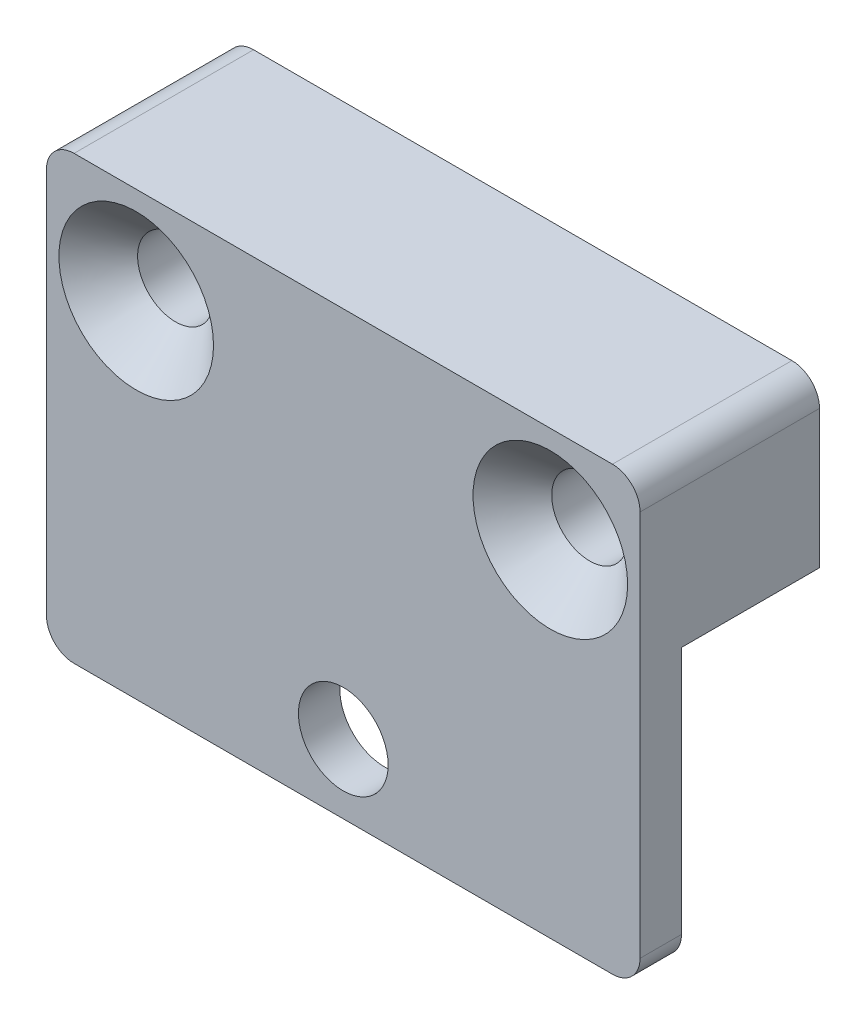
SolidWorks part; units mm, degrees
ref_plane "前视" through (0, 0, 0) normal (0, 0, 1) x (1, 0, 0)
ref_plane "上视" through (0, 0, 0) normal (0, 1, 0) x (1, 0, 0)
ref_plane "右视" through (0, 0, 0) normal (1, 0, 0) x (0, 0, -1)
sketch "草图1" plane through (0, 0, 0) normal (0, 0, 1) x (1, 0, 0)
  line L1 (0, 0) -> (43, 0)
  line L2 (0, 0) -> (0, -32)
  line L3 (0, -32) -> (43, -32)
  line L4 (43, 0) -> (43, -32)
  dimension "D1" = 43
  dimension "D2" = 32
extrude "凸台-拉伸1" add sketch "草图1" along normal blind 3
hole_wizard "M5 六角凹锥坑螺钉的锥形沉头孔1" positions "草图3" profile "草图2" countersink size "M5" standard "ISO" end condition through all
sketch "草图3" plane through (0, 0, 3) normal (0, 0, 1) x (1, 0, 0)
  line L0 (6.5, -7) -> (36.5, -7) construction
  line L2 (21.5, -7) -> (21.5, 0) construction
  line L3 (43, 0) -> (0, 0) construction
  point P0 (6.5, -7)
  point P2 (36.5, -7)
  dimension "D1" = 30
  dimension "D2" = 7
sketch "草图2" plane through (6.5, -7, 3) normal (1, 0, 0) x (0, -1, 0)
  line L0 (0, 0) -> (0, 3)
  line L1 (0, 3) -> (2.75, 3)
  line L2 (2.75, 3) -> (2.75, 2.85)
  line L3 (2.75, 2.85) -> (5.6, 0)
  line L5 (5.6, 0) -> (0, 0)
  line L6 (-2.75, 2.85) -> (-5.6, 0) construction
  line L11 (0, -6.35) -> (0, 107.95) construction
  dimension "通孔孔直径" = 5.5
  dimension "通孔孔深度" = 3
  dimension "近端锥形沉头孔直径" = 11.2
  dimension "近端锥形沉头孔角度" = 90
sketch "草图4" plane through (0, 0, 3) normal (0, 0, 1) x (1, 0, 0)
  line L0 (21.5, -32) -> (21.5, -27) construction
  line L1 (0, -32) -> (43, -32) construction
  circle A0 centre (21.5, -27) radius 3.25
  circle A1 centre (36.5, -7) radius 2.75 construction
  dimension "D1" = 6.5
  dimension "D2" = 20
extrude "切除-拉伸1" cut sketch "草图4" against normal blind 3
fillet "圆角1" radius 2 4 edges at (43, -32, 1.5) (0, -32, 1.5) (43, 0, 1.5) (0, 0, 1.5)
sketch "草图5" plane through (0, 0, 0) normal (0, 0, -1) x (-1, 0, 0)
  line L0 (-43, -12) -> (0, -12)
  line L4 (-2, 0) -> (-41, 0)
  line L5 (-43, -2) -> (-43, -30)
  line L6 (-41, -32) -> (-2, -32)
  line L7 (0, -30) -> (0, -2)
  line L8 (-2, 0) -> (-41, 0)
  line L9 (-43, -2) -> (-43, -30)
  line L10 (-41, -32) -> (-2, -32)
  line L11 (0, -30) -> (0, -2)
  arc A4 (-41, 0) -> (-43, -2) centre (-41, -2) ccw
  arc A5 (-43, -30) -> (-41, -32) centre (-41, -30) ccw
  arc A6 (-2, -32) -> (0, -30) centre (-2, -30) ccw
  arc A7 (0, -2) -> (-2, 0) centre (-2, -2) ccw
  arc A8 (-41, 0) -> (-43, -2) centre (-41, -2) ccw
  arc A9 (-43, -30) -> (-41, -32) centre (-41, -30) ccw
  arc A10 (-2, -32) -> (0, -30) centre (-2, -30) ccw
  arc A11 (0, -2) -> (-2, 0) centre (-2, -2) ccw
  circle M11 centre (-6.5, -7) radius 2.75
  circle M12 centre (-36.5, -7) radius 2.75
  line M13 (-2, 0) -> (-41, 0)
  arc M14 (-41, 0) -> (-43, -2) centre (-41, -2) ccw
  line M15 (-43, -2) -> (-43, -30)
  line M19 (0, -30) -> (0, -2)
  arc M20 (0, -2) -> (-2, 0) centre (-2, -2) ccw
  dimension "D2" = 12
  dimension "D1" = 0
extrude "凸台-拉伸2" add sketch "草图5" along normal blind 10 contours L0 M15 M19 M20 M13 M14 M12 M11
